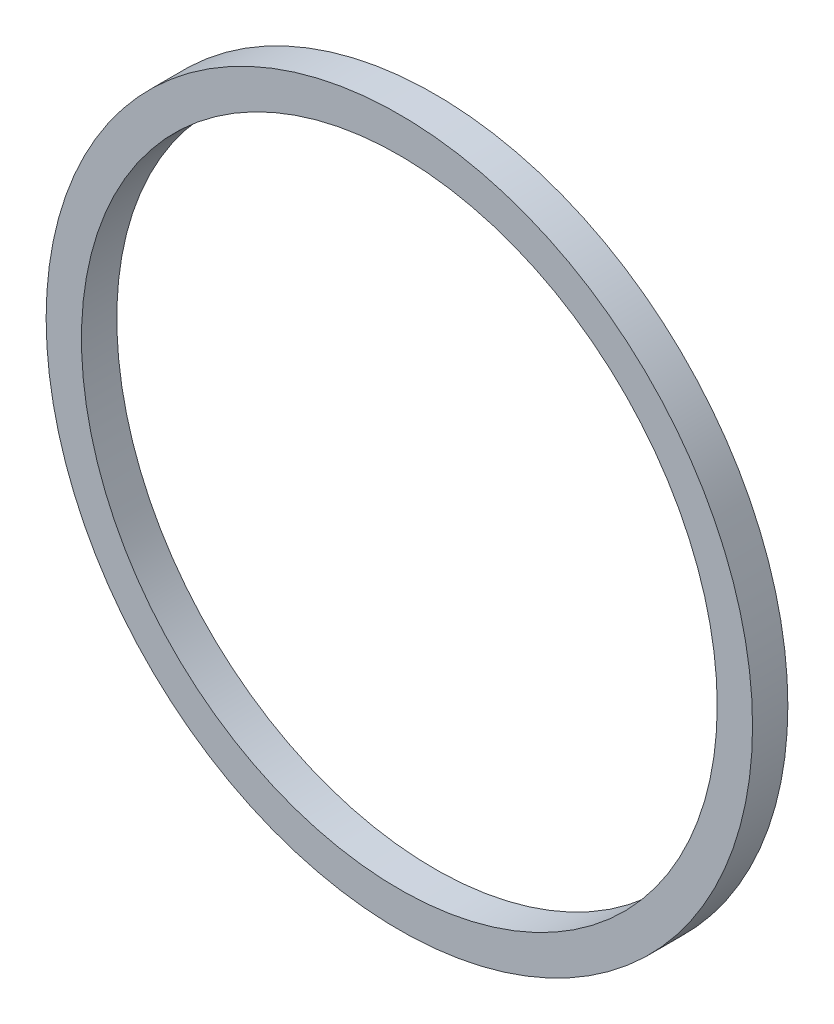
SolidWorks part; units mm, degrees
ref_plane "前视基准面" through (0, 0, 0) normal (0, 0, 1) x (1, 0, 0)
ref_plane "上视基准面" through (0, 0, 0) normal (0, 1, 0) x (1, 0, 0)
ref_plane "右视基准面" through (0, 0, 0) normal (1, 0, 0) x (0, 0, -1)
sketch "草图1" plane through (0, 0, 0) normal (0, 0, 1) x (1, 0, 0)
  circle A0 centre (0, 0) radius 30
  circle A1 centre (0, 0) radius 27
  dimension "D1" = 60
  dimension "D2" = 3
extrude "凸台-拉伸1" add sketch "草图1" along normal blind 3
equation "\"图号代码1\"= \"图号代码\""
equation "\"名称代码2\"= \"名称代码\""
